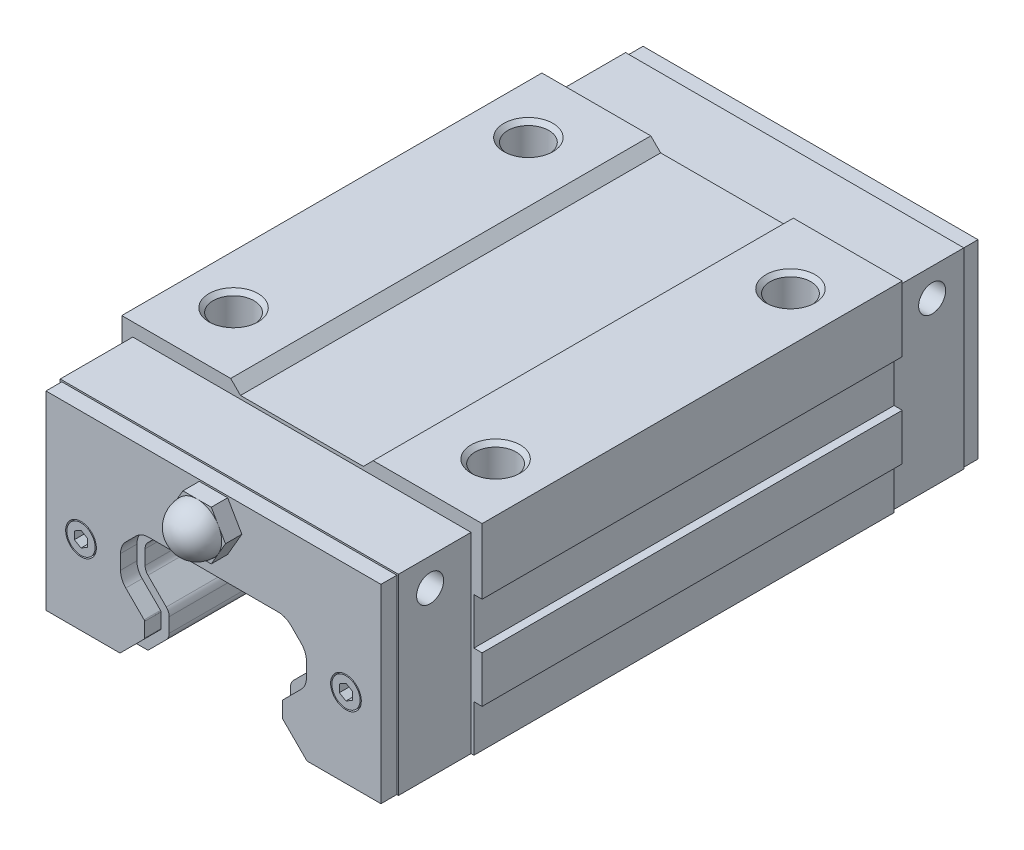
SolidWorks part; units mm, degrees
ref_plane "Front Plane" through (0, 0, 0) normal (0, 0, 1) x (1, 0, 0)
ref_plane "Top Plane" through (0, 0, 0) normal (0, 1, 0) x (1, 0, 0)
ref_plane "Right Plane" through (0, 0, 0) normal (1, 0, 0) x (0, 0, -1)
sketch "Sketch1" plane through (0, 0, 0) normal (0, 1, 0) x (1, 0, 0)
  line L1 (0, -36.45) -> (0, 36.45) construction
  line L2 (-22, -25.65) -> (22, -25.65)
  line L3 (-22, -25.65) -> (-22, 25.65)
  line L4 (-22, 25.65) -> (22, 25.65)
  line L5 (22, -25.65) -> (22, 25.65)
  line L6 (-22, 0) -> (22, 0) construction
  line L7 (22, -25.65) -> (22, -30.65) construction
  line L8 (0, -36.45) -> (0, -48.45) construction
  line L9 (22, 25.65) -> (22, 30.65) construction
  point P9 (-16, 18)
  point P12 (16, 18)
  point P13 (16, -18)
  point P14 (-16, -18)
  dimension "W" = 44
  dimension "L1" = 51.3
  dimension "L0" = 72.9
  dimension "B" = 32
  dimension "C" = 36
  dimension "K" = 5.8
  dimension "L2" = 12
sketch "Sketch2" plane through (0, 0, 0) normal (0, 0, 1) x (1, 0, 0)
  line L0 (-22, 0) -> (22, 0) construction
  line L1 (-22, 0) -> (22, 0)
  line L2 (-22, 0) -> (-22, 25)
  line L3 (-22, 25) -> (22, 25)
  line L4 (22, 0) -> (22, 25)
  line L5 (0, 0) -> (0, 25) construction
  line L6 (-22, 0) -> (-22, -5) construction
  line L7 (-10, -5) -> (10, -5)
  line L8 (-22, 23.4) -> (22, 23.4)
  line L9 (-10, -5) -> (-10, 0) construction
  line L10 (-10, 0) -> (-7.7627, 2.2373)
  line L11 (-7.4113, 3.0858) -> (-7.4113, 4.8515)
  line L12 (-7.7627, 5.7) -> (-10, 7.9373)
  line L13 (-10.3515, 8.7858) -> (-10.3515, 10.5515)
  line L14 (-10, 11.4) -> (-8.7515, 12.6485)
  line L15 (-7.9029, 13) -> (7.9029, 13)
  line L16 (10.3515, 8.7858) -> (10.3515, 10.5515)
  line L17 (7.7627, 5.7) -> (10, 7.9373)
  line L18 (7.4113, 3.0858) -> (7.4113, 4.8515)
  line L19 (10, 0) -> (7.7627, 2.2373)
  line L20 (10, 11.4) -> (8.7515, 12.6485)
  arc A0 (-7.7627, 2.2373) -> (-7.4113, 3.0858) centre (-8.6113, 3.0858) ccw
  arc A1 (-7.7627, 5.7) -> (-7.4113, 4.8515) centre (-8.6113, 4.8515) cw
  arc A2 (-10.3515, 8.7858) -> (-10, 7.9373) centre (-9.1515, 8.7858) ccw
  arc A3 (-10.3515, 10.5515) -> (-10, 11.4) centre (-9.1515, 10.5515) cw
  arc A4 (-8.7515, 12.6485) -> (-7.9029, 13) centre (-7.9029, 11.8) cw
  arc A5 (10.3515, 10.5515) -> (10, 11.4) centre (9.1515, 10.5515) ccw
  arc A6 (10.3515, 8.7858) -> (10, 7.9373) centre (9.1515, 8.7858) cw
  arc A7 (7.7627, 5.7) -> (7.4113, 4.8515) centre (8.6113, 4.8515) ccw
  arc A8 (7.7627, 2.2373) -> (7.4113, 3.0858) centre (8.6113, 3.0858) cw
  arc A9 (8.7515, 12.6485) -> (7.9029, 13) centre (7.9029, 11.8) ccw
  circle A10 centre (22, 20) radius 1.65
  point P9 (-22, 17)
  point P33 (-8.4, 13)
  point P50 (0, 13)
  dimension "D6" = 1.2
  dimension "(d1)" = 3.3
  dimension "D1" = 1.6
  dimension "H2" = 5
  dimension "H" = 30
  dimension "T" = 8
  dimension "D2" = 45
  dimension "W1" = 20
  dimension "D3" = 135
  dimension "H1" = 18
  dimension "D4" = 8.4
  dimension "D5" = 135
  dimension "N" = 5
sketch "Sketch3" plane through (0, 0, 0) normal (0, 0, 1) x (1, 0, 0)
  line L0 (-22, 23.4) -> (22, 23.4) construction
  line L1 (-22, 0) -> (-22, 25) construction
  line L14 (22, 0) -> (22, 25) construction
  line L15 (-22, 23.4) -> (22, 23.4)
  line L16 (-22, 0) -> (-22, 23.4)
  line L17 (-22, 0) -> (22, 0) construction
  line L18 (-22, 0) -> (22, 0)
  line L29 (22, 0) -> (22, 23.4)
extrude "Boss-Extrude1" add sketch "Sketch3" along normal up to vertex (36.45 mm away) from vertex at -36.45 starting at point (0, 0, -36.45)
sketch "Sketch5" plane through (0, 0, 0) normal (0, 1, 0) x (1, 0, 0)
  line L0 (-22, -25.65) -> (-22, 25.65) construction
  line L1 (-22, 25.65) -> (22, 25.65) construction
  line L2 (22, -25.65) -> (22, 25.65) construction
  line L3 (-22, -25.65) -> (22, -25.65) construction
  line L4 (-22, -25.65) -> (-22, 25.65)
  line L5 (-22, 25.65) -> (22, 25.65)
  line L6 (22, -25.65) -> (22, 25.65)
  line L7 (-22, -25.65) -> (22, -25.65)
extrude "凸台-拉伸1" add sketch "Sketch5" along normal up to vertex (25 mm away) up to point (0, 25, 0)
sketch "Sketch4" plane through (0, 0, 0) normal (0, 0, 1) x (1, 0, 0)
  line L0 (0, 0) -> (0, 13) construction
  line L1 (-22, 0) -> (-21, 0)
  line L2 (-22, 0) -> (-22, 17)
  line L3 (-22, 17) -> (-21, 17)
  line L4 (-21, 0) -> (-21, 17)
  line L5 (21, 0) -> (21, 17)
  line L6 (22, 17) -> (21, 17)
  line L7 (22, 0) -> (22, 5.6667)
  line L8 (22, 0) -> (21, 0)
  line L9 (-22, 0) -> (22, 0) construction
  line L10 (21, 11.3333) -> (22, 11.3333)
  line L11 (21, 5.6667) -> (22, 5.6667)
  line L12 (21, 8.5) -> (22, 8.5) construction
  line L13 (22, 11.3333) -> (22, 17)
  dimension "D1" = 1
  dimension "D2" = 5.6667
extrude "Cut-Extrude1" cut sketch "Sketch4" along normal up to vertex (36.45 mm away) from vertex at -36.45 contours L11 L5 L8 L7 | L10 L13 L6 L5 | L2 L3 L4 L1 starting at point (0, 0, -36.45)
sketch "Sketch6" plane through (0, 0, 25.65) normal (0, 0, 1) x (1, 0, 0)
  line L0 (0, 25) -> (0, 0) construction
  line L1 (-8.7, 25) -> (-7.5, 23.8)
  line L2 (-22, 25) -> (22, 25) construction
  line L3 (-7.5, 23.8) -> (7.5, 23.8)
  line L4 (7.5, 23.8) -> (8.7, 25)
  line L5 (-8.7, 25) -> (8.7, 25)
  dimension "D1" = 1.2
  dimension "D2" = 135
  dimension "D3" = 15
extrude "切除-拉伸1" cut sketch "Sketch6" against normal up to next
sketch "Sketch24" plane through (0, 0, 36.45) normal (0, 0, 1) x (1, 0, 0)
  line L0 (-22, 0) -> (22, 0) construction
  line L1 (-20.65, 0) -> (-22, 0)
  line L2 (-20.65, 0) -> (-20.65, 25)
  line L3 (-20.65, 25) -> (-22, 25)
  line L4 (-22, 0) -> (-22, 25)
  line L5 (20.65, 0) -> (22, 0)
  line L6 (20.65, 0) -> (20.65, 25)
  line L7 (20.65, 25) -> (22, 25)
  line L8 (22, 0) -> (22, 25)
  dimension "D1" = 1.35
  dimension "D2" = 1.35
extrude "Cut-Extrude6" cut sketch "Sketch24" against normal up to vertex (10.8 mm away)
sketch "Sketch25" plane through (0, 0, 36.45) normal (0, 0, 1) x (1, 0, 0)
  line L0 (-20.65, 0) -> (-20.65, 23.4) construction
  line L1 (-20.65, 23.4) -> (20.65, 23.4) construction
  line L2 (20.65, 23.4) -> (20.65, 0) construction
  line L3 (-20.65, 0) -> (-20.65, 23.4)
  line L4 (-20.65, 23.4) -> (20.65, 23.4)
  line L5 (20.65, 23.4) -> (20.65, 0)
  line L6 (-20.45, 0) -> (-20.45, 23.2)
  line L7 (-20.45, 23.2) -> (20.45, 23.2)
  line L8 (20.45, 23.2) -> (20.45, 0)
  line L9 (-20.65, 0) -> (-20.45, 0)
  line L10 (-20.45, 0) -> (-28.4625, 0.0015)
  line L11 (20.45, 0) -> (20.65, 0)
  dimension "D1" = 0.2
extrude "Cut-Extrude7" cut sketch "Sketch25" against normal blind 1.9333 contours L9 L3 L4 L5 L11 L8 L7 L6
sketch "Sketch7" plane through (0, 0, 0) normal (0, 0, 1) x (1, 0, 0)
  line L0 (-10, 0) -> (-7.7627, 2.2373) construction
  line L1 (-7.4113, 3.0858) -> (-7.4113, 4.8515) construction
  line L2 (-7.7627, 5.7) -> (-10, 7.9373) construction
  line L3 (-10.3515, 8.7858) -> (-10.3515, 10.5515) construction
  line L4 (-10, 11.4) -> (-8.7515, 12.6485) construction
  line L5 (-7.9029, 13) -> (7.9029, 13) construction
  line L6 (10, 11.4) -> (8.7515, 12.6485) construction
  line L7 (10.3515, 8.7858) -> (10.3515, 10.5515) construction
  line L8 (7.7627, 5.7) -> (10, 7.9373) construction
  line L9 (7.4113, 3.0858) -> (7.4113, 4.8515) construction
  line L10 (10, 0) -> (7.7627, 2.2373) construction
  line L11 (-10, 0) -> (-7.7627, 2.2373)
  line L12 (-7.4113, 3.0858) -> (-7.4113, 4.8515)
  line L13 (-7.7627, 5.7) -> (-10, 7.9373)
  line L14 (-10.3515, 8.7858) -> (-10.3515, 10.5515)
  line L15 (-10, 11.4) -> (-8.7515, 12.6485)
  line L16 (-7.9029, 13) -> (7.9029, 13)
  line L17 (10, 11.4) -> (8.7515, 12.6485)
  line L18 (10.3515, 8.7858) -> (10.3515, 10.5515)
  line L19 (7.7627, 5.7) -> (10, 7.9373)
  line L20 (7.4113, 3.0858) -> (7.4113, 4.8515)
  line L21 (10, 0) -> (7.7627, 2.2373)
  line L22 (-10, 0) -> (10, 0)
  arc A0 (-7.7627, 2.2373) -> (-7.4113, 3.0858) centre (-8.6113, 3.0858) ccw construction
  arc A1 (-7.4113, 4.8515) -> (-7.7627, 5.7) centre (-8.6113, 4.8515) ccw construction
  arc A2 (-10.3515, 8.7858) -> (-10, 7.9373) centre (-9.1515, 8.7858) ccw construction
  arc A3 (-10, 11.4) -> (-10.3515, 10.5515) centre (-9.1515, 10.5515) ccw construction
  arc A4 (-7.9029, 13) -> (-8.7515, 12.6485) centre (-7.9029, 11.8) ccw construction
  arc A5 (8.7515, 12.6485) -> (7.9029, 13) centre (7.9029, 11.8) ccw construction
  arc A6 (10.3515, 10.5515) -> (10, 11.4) centre (9.1515, 10.5515) ccw construction
  arc A7 (10, 7.9373) -> (10.3515, 8.7858) centre (9.1515, 8.7858) ccw construction
  arc A8 (7.7627, 5.7) -> (7.4113, 4.8515) centre (8.6113, 4.8515) ccw construction
  arc A9 (7.4113, 3.0858) -> (7.7627, 2.2373) centre (8.6113, 3.0858) ccw construction
  arc A10 (-7.7627, 2.2373) -> (-7.4113, 3.0858) centre (-8.6113, 3.0858) ccw
  arc A11 (-7.4113, 4.8515) -> (-7.7627, 5.7) centre (-8.6113, 4.8515) ccw
  arc A12 (-10.3515, 8.7858) -> (-10, 7.9373) centre (-9.1515, 8.7858) ccw
  arc A13 (-10, 11.4) -> (-10.3515, 10.5515) centre (-9.1515, 10.5515) ccw
  arc A14 (-7.9029, 13) -> (-8.7515, 12.6485) centre (-7.9029, 11.8) ccw
  arc A15 (8.7515, 12.6485) -> (7.9029, 13) centre (7.9029, 11.8) ccw
  arc A16 (10.3515, 10.5515) -> (10, 11.4) centre (9.1515, 10.5515) ccw
  arc A17 (10, 7.9373) -> (10.3515, 8.7858) centre (9.1515, 8.7858) ccw
  arc A18 (7.7627, 5.7) -> (7.4113, 4.8515) centre (8.6113, 4.8515) ccw
  arc A19 (7.4113, 3.0858) -> (7.7627, 2.2373) centre (8.6113, 3.0858) ccw
extrude "Cut-Extrude2" cut sketch "Sketch7" against normal up to vertex (36.45 mm away) from vertex at 36.45 starting at point (0, 0, 36.45)
sketch "Sketch8" plane through (0, 0, 36.45) normal (0, 0, 1) x (1, 0, 0)
  line L0 (-7.7627, 2.2373) -> (-10, 0) construction
  line L1 (-7.4113, 4.8515) -> (-7.4113, 3.0858) construction
  line L2 (-10, 7.9373) -> (-7.7627, 5.7) construction
  line L3 (-10.3515, 10.5515) -> (-10.3515, 8.7858) construction
  line L4 (-8.7515, 12.6485) -> (-10, 11.4) construction
  line L5 (7.9029, 13) -> (-7.9029, 13) construction
  line L6 (10, 11.4) -> (8.7515, 12.6485) construction
  line L7 (10.3515, 8.7858) -> (10.3515, 10.5515) construction
  line L8 (7.7627, 5.7) -> (10, 7.9373) construction
  line L9 (7.4113, 3.0858) -> (7.4113, 4.8515) construction
  line L10 (10, 0) -> (7.7627, 2.2373) construction
  line L11 (-7.7627, 2.2373) -> (-10, 0)
  line L12 (-7.4113, 4.8515) -> (-7.4113, 3.0858)
  line L13 (-10, 7.9373) -> (-7.7627, 5.7)
  line L14 (-10.3515, 10.5515) -> (-10.3515, 8.7858)
  line L15 (-8.7515, 12.6485) -> (-10, 11.4)
  line L16 (7.9029, 13) -> (-7.9029, 13)
  line L17 (10, 11.4) -> (8.7515, 12.6485)
  line L18 (10.3515, 8.7858) -> (10.3515, 10.5515)
  line L19 (7.7627, 5.7) -> (10, 7.9373)
  line L20 (7.4113, 3.0858) -> (7.4113, 4.8515)
  line L21 (10, 0) -> (7.7627, 2.2373)
  line L22 (10.7071, 0.7071) -> (8.4698, 2.9444)
  line L23 (8.4113, 3.0858) -> (8.4113, 4.8515)
  line L24 (8.4698, 4.9929) -> (10.7071, 7.2302)
  line L25 (11.3515, 8.7858) -> (11.3515, 10.5515)
  line L26 (10.7071, 12.1071) -> (9.4586, 13.3556)
  line L27 (7.9029, 14) -> (-7.9029, 14)
  line L28 (-9.4586, 13.3556) -> (-10.7071, 12.1071)
  line L29 (-11.3515, 10.5515) -> (-11.3515, 8.7858)
  line L30 (-10.7071, 7.2302) -> (-8.4698, 4.9929)
  line L31 (-8.4113, 4.8515) -> (-8.4113, 3.0858)
  line L32 (-8.4698, 2.9444) -> (-10.7071, 0.7071)
  line L33 (-10.7071, 0.7071) -> (-11.4142, 0)
  line L34 (-22, 0) -> (22, 0) construction
  line L35 (-11.4142, 0) -> (-10, 0)
  line L36 (10.7071, 0.7071) -> (11.4142, 0)
  line L37 (-22, 0) -> (22, 0) construction
  line L38 (11.4142, 0) -> (10, 0)
  arc A0 (-7.7627, 2.2373) -> (-7.4113, 3.0858) centre (-8.6113, 3.0858) ccw construction
  arc A1 (-7.4113, 4.8515) -> (-7.7627, 5.7) centre (-8.6113, 4.8515) ccw construction
  arc A2 (-10.3515, 8.7858) -> (-10, 7.9373) centre (-9.1515, 8.7858) ccw construction
  arc A3 (-10, 11.4) -> (-10.3515, 10.5515) centre (-9.1515, 10.5515) ccw construction
  arc A4 (-7.9029, 13) -> (-8.7515, 12.6485) centre (-7.9029, 11.8) ccw construction
  arc A5 (8.7515, 12.6485) -> (7.9029, 13) centre (7.9029, 11.8) ccw construction
  arc A6 (10.3515, 10.5515) -> (10, 11.4) centre (9.1515, 10.5515) ccw construction
  arc A7 (10, 7.9373) -> (10.3515, 8.7858) centre (9.1515, 8.7858) ccw construction
  arc A8 (7.7627, 5.7) -> (7.4113, 4.8515) centre (8.6113, 4.8515) ccw construction
  arc A9 (7.4113, 3.0858) -> (7.7627, 2.2373) centre (8.6113, 3.0858) ccw construction
  arc A10 (-7.7627, 2.2373) -> (-7.4113, 3.0858) centre (-8.6113, 3.0858) ccw
  arc A11 (-7.4113, 4.8515) -> (-7.7627, 5.7) centre (-8.6113, 4.8515) ccw
  arc A12 (-10.3515, 8.7858) -> (-10, 7.9373) centre (-9.1515, 8.7858) ccw
  arc A13 (-10, 11.4) -> (-10.3515, 10.5515) centre (-9.1515, 10.5515) ccw
  arc A14 (-7.9029, 13) -> (-8.7515, 12.6485) centre (-7.9029, 11.8) ccw
  arc A15 (8.7515, 12.6485) -> (7.9029, 13) centre (7.9029, 11.8) ccw
  arc A16 (10.3515, 10.5515) -> (10, 11.4) centre (9.1515, 10.5515) ccw
  arc A17 (10, 7.9373) -> (10.3515, 8.7858) centre (9.1515, 8.7858) ccw
  arc A18 (7.7627, 5.7) -> (7.4113, 4.8515) centre (8.6113, 4.8515) ccw
  arc A19 (7.4113, 3.0858) -> (7.7627, 2.2373) centre (8.6113, 3.0858) ccw
  arc A20 (8.4113, 3.0858) -> (8.4698, 2.9444) centre (8.6113, 3.0858) ccw
  arc A21 (8.4698, 4.9929) -> (8.4113, 4.8515) centre (8.6113, 4.8515) ccw
  arc A22 (10.7071, 7.2302) -> (11.3515, 8.7858) centre (9.1515, 8.7858) ccw
  arc A23 (11.3515, 10.5515) -> (10.7071, 12.1071) centre (9.1515, 10.5515) ccw
  arc A24 (9.4586, 13.3556) -> (7.9029, 14) centre (7.9029, 11.8) ccw
  arc A25 (-7.9029, 14) -> (-9.4586, 13.3556) centre (-7.9029, 11.8) ccw
  arc A26 (-10.7071, 12.1071) -> (-11.3515, 10.5515) centre (-9.1515, 10.5515) ccw
  arc A27 (-11.3515, 8.7858) -> (-10.7071, 7.2302) centre (-9.1515, 8.7858) ccw
  arc A28 (-8.4113, 4.8515) -> (-8.4698, 4.9929) centre (-8.6113, 4.8515) ccw
  arc A29 (-8.4698, 2.9444) -> (-8.4113, 3.0858) centre (-8.6113, 3.0858) ccw
  dimension "D1" = 1
extrude "Cut-Extrude3" cut sketch "Sketch8" against normal blind 2
mirror "Mirror1" about plane through (0, 0, 0) normal (0, 0, 1) of "Cut-Extrude7", "Cut-Extrude3", "Cut-Extrude6"
hole_wizard "threaded hole 1" positions "Sketch18" profile "Sketch17" tap size "M8" standard "GB"
sketch "Sketch18" plane through (0, 25, 0) normal (0, 1, 0) x (-1, 0, 0)
  point P0 (16, 18)
  point P3 (-16, -18)
  point P5 (16, -18)
  point P7 (-16, 18)
sketch "Sketch17" plane through (-16, 25, 18) normal (1, 0, 0) x (0, 0, 1)
  line L0 (0, 0) -> (0, 7.5022)
  line L1 (0, 7.5022) -> (2.5, 6)
  line L2 (2.5, 6) -> (2.5, 0)
  line L5 (2.5, 0) -> (0, 0)
  line L10 (0, 7.5022) -> (-2.5, 6) construction
  line L11 (0, -6.35) -> (0, 7.5022) construction
  dimension "S" = 5
  dimension "ℓ" = 6
  dimension "导头角度" = 118
cosmetic thread "Hole Cosmetic Thread1" parameters "D1"=16, "D2"=5
cosmetic thread "Hole Cosmetic Thread2" parameters "D1"=16, "D2"=5
cosmetic thread "Hole Cosmetic Thread3" parameters "D1"=16, "D2"=5
cosmetic thread "Hole Cosmetic Thread4" parameters "D1"=16, "D2"=5
chamfer "Chamfer1" distance 0.5 angle 45 4 edges at (16, 25, -15.5) (16, 25, 20.5) (-16, 25, 20.5) (-16, 25, -15.5)
sketch "Sketch19" plane through (0, 0, 36.45) normal (0, 0, 1) x (1, 0, 0)
  line L0 (-11.3515, 9.6686) -> (-21, 9.6686) construction
  line L1 (-11.3515, 10.5515) -> (-11.3515, 8.7858) construction
  line L2 (-21, 17) -> (-21, 0) construction
  line L3 (0, 0) -> (0, 13) construction
  line L4 (-7.9029, 13) -> (7.9029, 13) construction
  line L5 (-16.1757, 10.6061) -> (-16.1757, 11.5436) construction
  line L6 (-16.1757, 9.6686) -> (-16.1757, 10.6061) construction
  line L7 (-16.1757, 10.6061) -> (-16.9876, 10.1374)
  line L8 (-16.9876, 10.1374) -> (-16.9876, 9.1999)
  line L9 (-16.9876, 9.1999) -> (-16.1757, 8.7311)
  line L10 (-16.1757, 8.7311) -> (-15.3638, 9.1999)
  line L11 (-15.3638, 9.1999) -> (-15.3638, 10.1374)
  line L12 (-15.3638, 10.1374) -> (-16.1757, 10.6061)
  line L13 (-16.1757, 7.7936) -> (-16.1757, 7.9436) construction
  line L14 (16.1757, 7.7936) -> (16.1757, 7.9436) construction
  line L15 (16.1757, 9.6686) -> (16.1757, 10.6061) construction
  line L16 (16.1757, 10.6061) -> (16.1757, 11.5436) construction
  line L17 (11.3515, 9.6686) -> (21, 9.6686) construction
  line L18 (15.3638, 10.1374) -> (16.1757, 10.6061)
  line L19 (15.3638, 9.1999) -> (15.3638, 10.1374)
  line L20 (16.1757, 8.7311) -> (15.3638, 9.1999)
  line L21 (16.9876, 9.1999) -> (16.1757, 8.7311)
  line L22 (16.9876, 10.1374) -> (16.9876, 9.1999)
  line L23 (16.1757, 10.6061) -> (16.9876, 10.1374)
  circle A0 centre (-16.1757, 9.6686) radius 1.875
  circle A1 centre (-16.1757, 9.6686) radius 1.725
  circle A2 centre (-16.1757, 9.6686) radius 0.8119 construction
  circle A3 centre (16.1757, 9.6686) radius 0.8119 construction
  circle A4 centre (16.1757, 9.6686) radius 1.725
  circle A5 centre (16.1757, 9.6686) radius 1.875
  dimension "D1" = 3.75
  dimension "D2" = 0.15
extrude "Cut-Extrude4" cut sketch "Sketch19" against normal blind 2 contours L11 L12 L7 L8 L9 L10 | A0 A1 | L23 L18 L19 L20 L21 L22 | A5 A4
mirror "Mirror2" about plane through (0, 0, 0) normal (0, 0, 1) of "Cut-Extrude4"
sketch "Sketch20" plane through (21, 0, 0) normal (1, 0, 0) x (0, 0, -1)
  circle A0 centre (-30.65, 20) radius 1.65
  circle A1 centre (30.65, 20) radius 1.65
  dimension "D1" = 3.3
extrude "Cut-Extrude5" cut sketch "Sketch20" against normal blind 3
sketch "Sketch22" plane through (0, 0, 36.45) normal (0, 0, 1) x (1, 0, 0)
  line L0 (0, 13) -> (0, 23.4) construction
  line L1 (1.7321, 23) -> (-1.7321, 23)
  line L2 (-1.7321, 23) -> (-3.4641, 20)
  line L3 (-3.4641, 20) -> (-1.7321, 17)
  line L4 (-1.7321, 17) -> (1.7321, 17)
  line L5 (1.7321, 17) -> (3.4641, 20)
  line L6 (3.4641, 20) -> (1.7321, 23)
  line L7 (-7.9029, 13) -> (7.9029, 13) construction
  line L8 (21, 23.4) -> (-21, 23.4) construction
  circle A0 centre (0, 20) radius 3 construction
  dimension "油嘴规格" = 6
extrude "Boss-Extrude2" add sketch "Sketch22" along normal blind 2
sketch "Sketch23" plane through (0, 0, 0) normal (1, 0, 0) x (0, 0, -1)
  line L0 (-38.45, 20) -> (-54.1488, 20) construction
  line L2 (-38.45, 20) -> (-38.45, 23)
  line L3 (-38.45, 17) -> (-38.45, 20) construction
  line L4 (-41.45, 20) -> (-38.45, 20)
  arc A0 (-38.45, 23) -> (-41.45, 20) centre (-38.45, 20) ccw
revolve "Revolve1" add sketch "Sketch23" angle 360 about L0
mirror "Mirror3" about plane through (0, 0, 0) normal (1, 0, 0) of "Cut-Extrude5"
